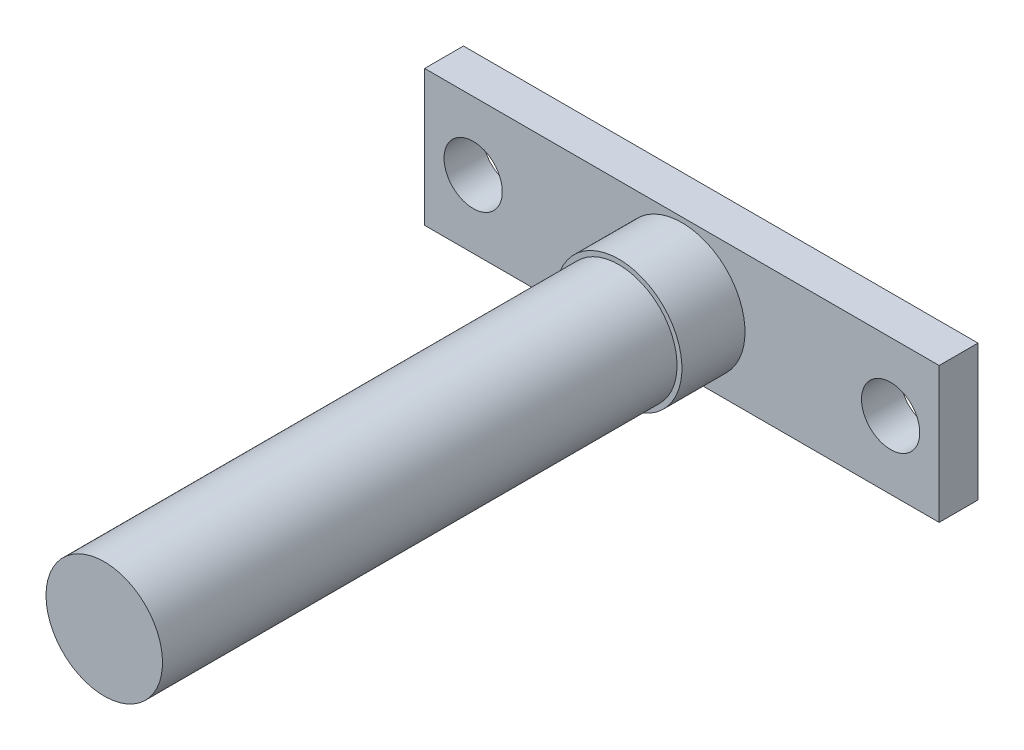
from build123d import *

# Parameters (mm, degrees)
SKETCH_1_R      = 6
EXTRUDE_1_DEPTH = 59.5
SKETCH_2_W      = 53
SKETCH_2_H      = 14
SKETCH_2_R      = 3
EXTRUDE_2_DEPTH = 4
SKETCH_3_R      = 6.5
EXTRUDE_3_DEPTH = 6.5


with BuildPart() as part:
    # 草图1 → 凸台-拉伸1 (new body)
    with BuildSketch(Plane.XY):
        with Locations(Location((0, 0, 0), (0, 0, 180))):
            Circle(SKETCH_1_R)
    extrude(amount=EXTRUDE_1_DEPTH)

    # 草图2 → 凸台-拉伸2 (add)
    with BuildSketch(Plane(origin=(0, 0, 0), x_dir=(-1, 0, 0), z_dir=(0, 0, -1))):
        Rectangle(SKETCH_2_W, SKETCH_2_H)
        with Locations((-21.5, 0)):
            Circle(SKETCH_2_R, mode=Mode.SUBTRACT)
        with Locations((21.5, 0)):
            Circle(SKETCH_2_R, mode=Mode.SUBTRACT)
    extrude(amount=EXTRUDE_2_DEPTH)

    # 草图3 → 凸台-拉伸3 (add)
    with BuildSketch(Plane.XY):
        with Locations(Location((0, 0, 0), (0, 0, 180))):
            Circle(SKETCH_3_R)
    extrude(amount=EXTRUDE_3_DEPTH)


solid = part.part
